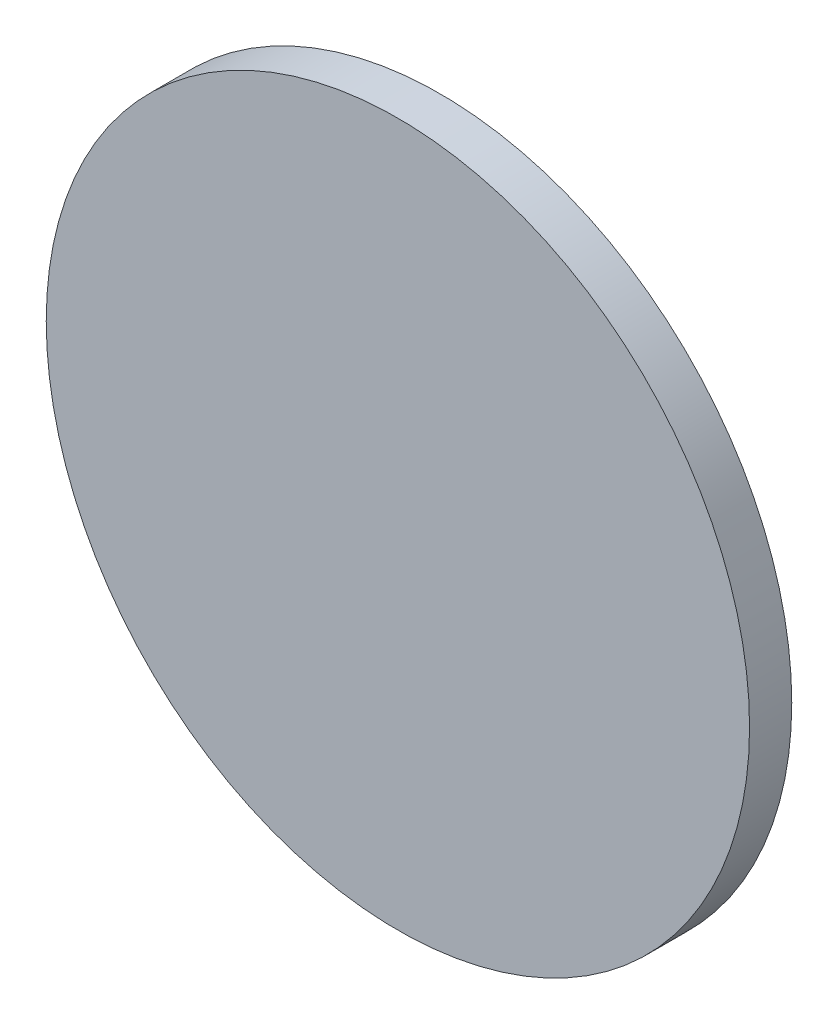
from build123d import *

# Parameters (mm, degrees)
SKETCH1_R           = 25
BOSS_EXTRUDE1_DEPTH = 3


with BuildPart() as part:
    # Sketch1 → Boss-Extrude1 (new body)
    with BuildSketch(Plane.XY):
        Circle(SKETCH1_R)
    extrude(amount=BOSS_EXTRUDE1_DEPTH)


solid = part.part
